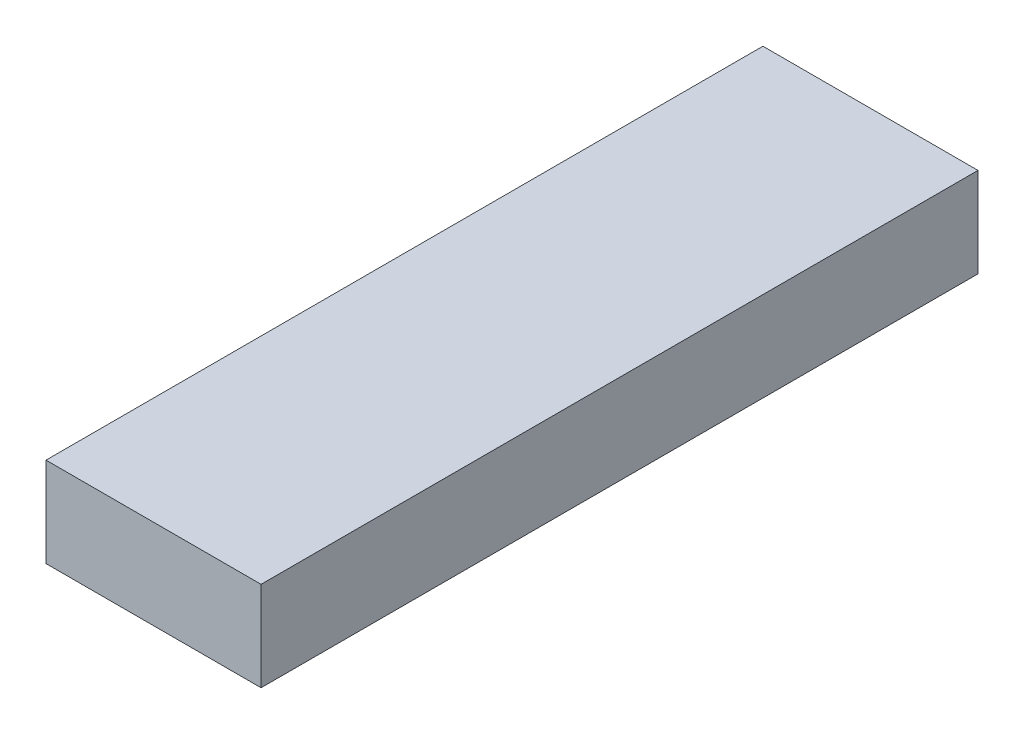
from build123d import *

# Parameters (mm, degrees)
SKETCH1_W           = 120
SKETCH1_H           = 50
BOSS_EXTRUDE1_DEPTH = 400


with BuildPart() as part:
    # Sketch1 → Boss-Extrude1 (new body)
    with BuildSketch(Plane.XY):
        with Locations((60, 25)):
            Rectangle(SKETCH1_W, SKETCH1_H)
    extrude(amount=BOSS_EXTRUDE1_DEPTH)


solid = part.part
